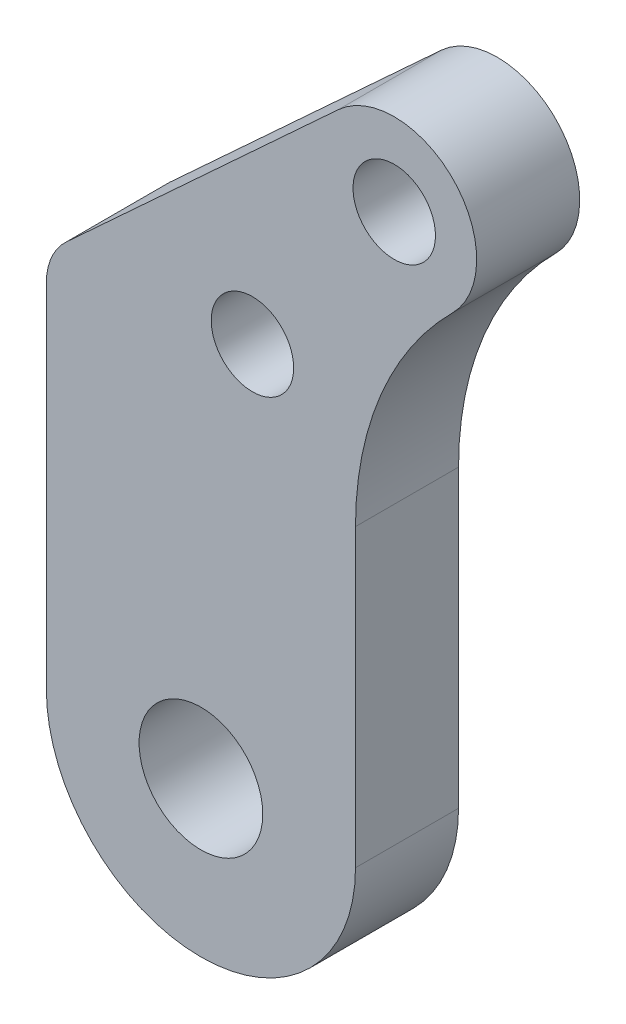
SolidWorks part; units mm, degrees
ref_plane "Front Plane" through (0, 0, 0) normal (0, 0, 1) x (1, 0, 0)
ref_plane "Top Plane" through (0, 0, 0) normal (0, 1, 0) x (1, 0, 0)
ref_plane "Right Plane" through (0, 0, 0) normal (1, 0, 0) x (0, 0, -1)
other "Configuration Table"
sketch "Sketch1" plane through (0, 0, 0) normal (0, 0, 1) x (1, 0, 0)
  line L0 (-7.5, 0) -> (-7.5, 17.0739)
  line L1 (-6.5326, 19.2804) -> (6.6699, 31.442)
  line L2 (7.5, 0) -> (7.5, 14.3358)
  circle A0 centre (0, 0) radius 3
  arc A1 (-7.5, 0) -> (7.5, 0) centre (0, 0) ccw
  circle A2 centre (2.5, 19.5) radius 2
  circle A3 centre (9.38, 28.5) radius 2
  arc A4 (12.204, 25.6672) -> (6.6699, 31.442) centre (9.38, 28.5) ccw
  arc A5 (12.204, 25.6672) -> (7.5, 14.3358) centre (23.5, 14.3358) ccw
  arc A6 (-6.5326, 19.2804) -> (-7.5, 17.0739) centre (-4.5, 17.0739) ccw
  dimension "D1" = 15
  dimension "D2" = 6
  dimension "D4" = 4
  dimension "D6" = 9.38
  dimension "D7" = 28.5
  dimension "D8" = 19.5
  dimension "D9" = 4
  dimension "D10" = 8
  dimension "D11" = 32
  dimension "D12" = 3
  dimension "D3" = 2.5
  dimension "D5" = 47.35
extrude "Boss-Extrude1" add sketch "Sketch1" along normal blind 5
